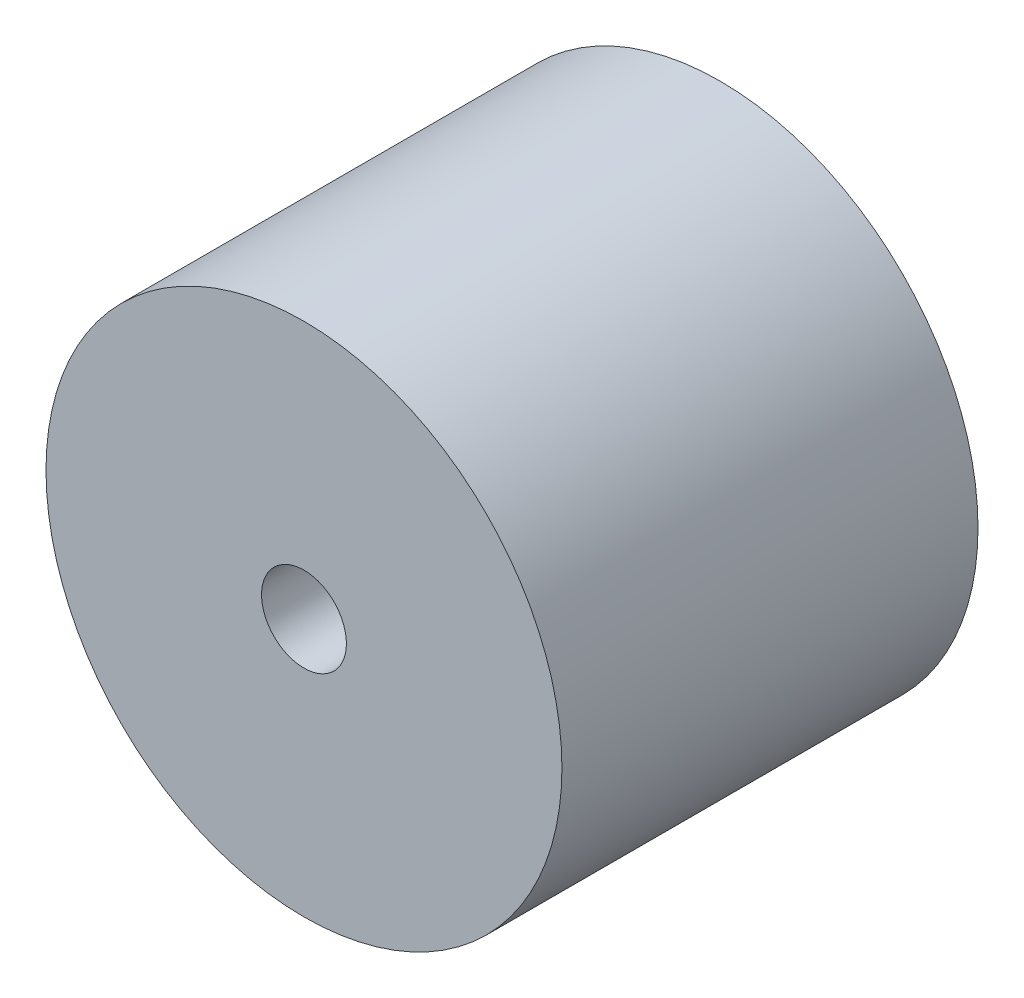
from build123d import *

# Parameters (mm, degrees)
SKETCH1_R              = 31
BOSS_EXTRUDE1_DEPTH    = 50
M12_TAPPED_HOLE1_D     = 10.2
M12_TAPPED_HOLE1_DEPTH = 29.25
M12_TAPPED_HOLE1_TIP   = 3.064389157


with BuildPart() as part:
    # Sketch1 → Boss-Extrude1 (new body)
    with BuildSketch(Plane.XY):
        Circle(SKETCH1_R)
    extrude(amount=BOSS_EXTRUDE1_DEPTH)

    # M12 Tapped Hole1
    with Locations(Plane.XY.offset(50)):
        with Locations((0, 0)):
            Hole(M12_TAPPED_HOLE1_D / 2, depth=M12_TAPPED_HOLE1_DEPTH)
            with Locations((0, 0, -(M12_TAPPED_HOLE1_DEPTH + M12_TAPPED_HOLE1_TIP / 2))):  # 118° drill point
                Cone(0, M12_TAPPED_HOLE1_D / 2, M12_TAPPED_HOLE1_TIP, mode=Mode.SUBTRACT)


solid = part.part
